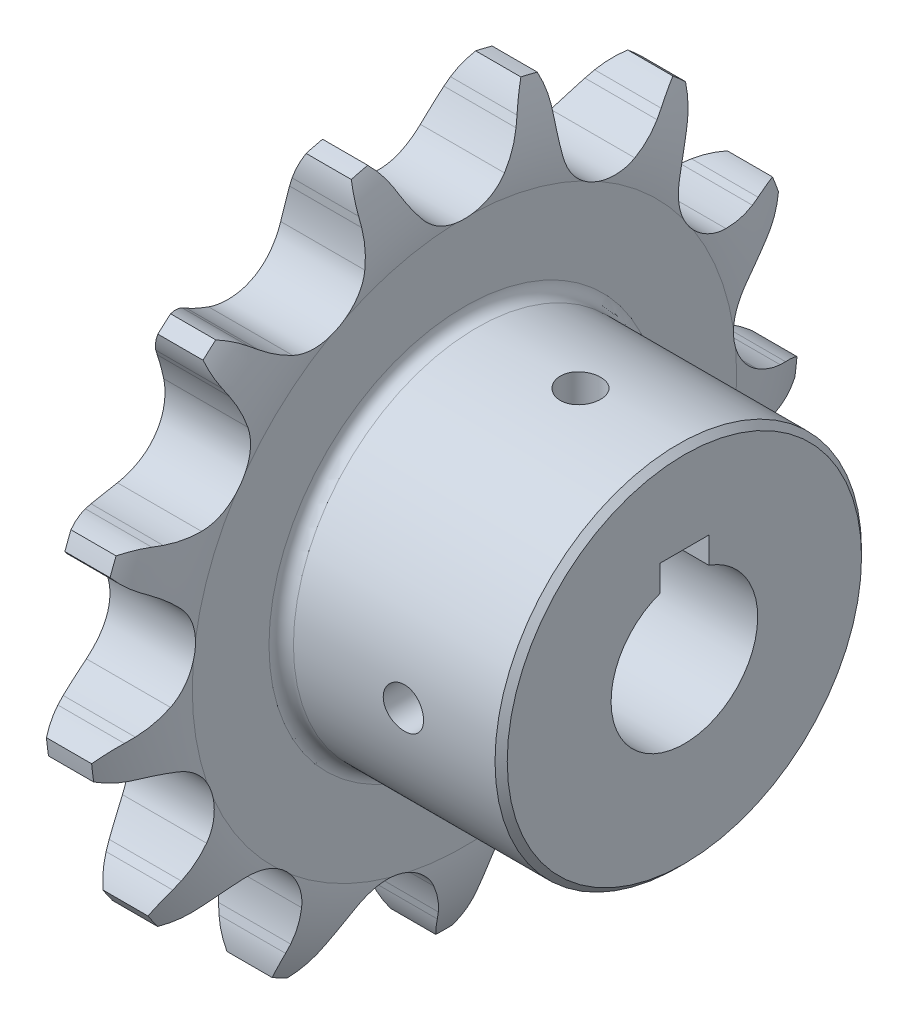
from build123d import *

# Parameters (mm, degrees)
CUT_EXTRUDE_1_DEPTH      = 4.638656443
PATTERN_CIRCULAR_1_COUNT = 13
SKETCH_3_R               = 15
SKETCH_3_R_2             = 6
EXTRUDE_1_DEPTH          = 18
FILLET_1_R               = 1
CHAMFER_1_SIZE           = 0.5
HOLE_WIZARD_M4_1_D       = 3.3
HOLE_WIZARD_M4_1_DEPTH   = 15
HOLE_WIZARD_M4_1_TIP     = 0.991420021
HOLE_WIZARD_M4_2_D       = 3.3
HOLE_WIZARD_M4_2_DEPTH   = 14.1
HOLE_WIZARD_M4_2_TIP     = 0.991420021
SKETCH_9_W               = 4
SKETCH_9_H               = 3.6
CUT_EXTRUDE_2_DEPTH      = 47


with BuildPart() as part:
    # 草图1 → 旋转1 (revolve)
    with BuildSketch(Plane.XY, mode=Mode.PRIVATE) as revolve_1_sk:
        with BuildLine():
            Line((-3.5, 6), (-3.5, 22.278992327))
            ThreePointArc((-3.5, 22.278992327), (-3.141151912, 25.754128127), (-1.849, 29))
            Line((-1.849, 29), (1.849, 29))
            ThreePointArc((1.849, 29), (3.141151912, 25.754128127), (3.5, 22.278992327))
            Line((3.5, 22.278992327), (3.5, 6))
            Line((3.5, 6), (-3.5, 6))
        make_face()
    revolve(revolve_1_sk.sketch.rotate(Axis((-6.35, 0, 0), (1, 0, 0)), 90), axis=Axis((-6.35, 0, 0), (1, 0, 0)))

    # 草图2 → 切除-拉伸1 (cut, symmetric)
    with BuildSketch(Plane(origin=(0, 0, 0), x_dir=(0, 0, -1), z_dir=(1, 0, 0))):
        with BuildLine():
            Line((4.769475288, 26.007478281), (5.07686592, 26.639875941))
            ThreePointArc((5.07686592, 26.639875941), (5.601425484, 27.526379428), (6.263467786, 28.31552527))
            ThreePointArc((6.263467786, 28.31552527), (0, 29), (-6.263467786, 28.31552527))
            ThreePointArc((-6.263467786, 28.31552527), (-5.601425484, 27.526379428), (-5.07686592, 26.639875941))
            Line((-5.07686592, 26.639875941), (-4.769475288, 26.007478281))
            ThreePointArc((-4.769475288, 26.007478281), (-4.11784871, 24.848481966), (-3.332711591, 23.775425883))
            ThreePointArc((-3.332711591, 23.775425883), (0, 22.207717327), (3.332711591, 23.775425883))
            ThreePointArc((3.332711591, 23.775425883), (4.11784871, 24.848481966), (4.769475288, 26.007478281))
        make_face()
    cut_extrude_1 = extrude(amount=CUT_EXTRUDE_1_DEPTH, both=True, mode=Mode.SUBTRACT)

    # 阵列(圆周)1: 切除-拉伸1 ×13 about axis
    pattern_circular_1_axis = Axis((0, 0, 0), (1, 0, 0))
    for i in range(1, PATTERN_CIRCULAR_1_COUNT):
        add(cut_extrude_1.rotate(pattern_circular_1_axis, i * 360 / PATTERN_CIRCULAR_1_COUNT), mode=Mode.SUBTRACT)

    # 草图3 → 凸台-拉伸1 (add)
    with BuildSketch(Plane(origin=(3.5, 0, 0), x_dir=(0, 0, -1), z_dir=(1, 0, 0))):
        with Locations(Location((0, 0, 0), (0, 0, 180))):
            Circle(SKETCH_3_R)
        with Locations(Location((0, 0, 0), (0, 0, 180))):
            Circle(SKETCH_3_R_2, mode=Mode.SUBTRACT)
    extrude(amount=EXTRUDE_1_DEPTH)

    # 圆角1
    fillet_1_edges = [part.edges().sort_by_distance(p)[0] for p in [
        (3.5, 0, -15),
    ]]
    fillet(fillet_1_edges, radius=FILLET_1_R)

    # 倒角1
    chamfer_1_edges = [part.edges().sort_by_distance(p)[0] for p in [
        (21.5, 0, -15),
    ]]
    chamfer(chamfer_1_edges, length=CHAMFER_1_SIZE)

    # M4 螺纹孔1
    with Locations(Plane(origin=(0, 17.5, 0), x_dir=(1, 0, 0), z_dir=(0, 1, 0))):
        with Locations((13, 0)):
            Hole(HOLE_WIZARD_M4_1_D / 2, depth=HOLE_WIZARD_M4_1_DEPTH)
            with Locations((0, 0, -(HOLE_WIZARD_M4_1_DEPTH + HOLE_WIZARD_M4_1_TIP / 2))):  # 118° drill point
                Cone(0, HOLE_WIZARD_M4_1_D / 2, HOLE_WIZARD_M4_1_TIP, mode=Mode.SUBTRACT)

    # M4 螺纹孔2
    with Locations(Plane.XY.offset(17.5)):
        with Locations((13.5, 0)):
            Hole(HOLE_WIZARD_M4_2_D / 2, depth=HOLE_WIZARD_M4_2_DEPTH)
            with Locations((0, 0, -(HOLE_WIZARD_M4_2_DEPTH + HOLE_WIZARD_M4_2_TIP / 2))):  # 118° drill point
                Cone(0, HOLE_WIZARD_M4_2_D / 2, HOLE_WIZARD_M4_2_TIP, mode=Mode.SUBTRACT)

    # 草图9 → 切除-拉伸2 (cut)
    with BuildSketch(Plane(origin=(21.5, 0, 0), x_dir=(0, 0, -1), z_dir=(1, 0, 0))):
        with Locations((0, 6)):
            Rectangle(SKETCH_9_W, SKETCH_9_H)
    extrude(amount=-CUT_EXTRUDE_2_DEPTH, mode=Mode.SUBTRACT)


solid = part.part
